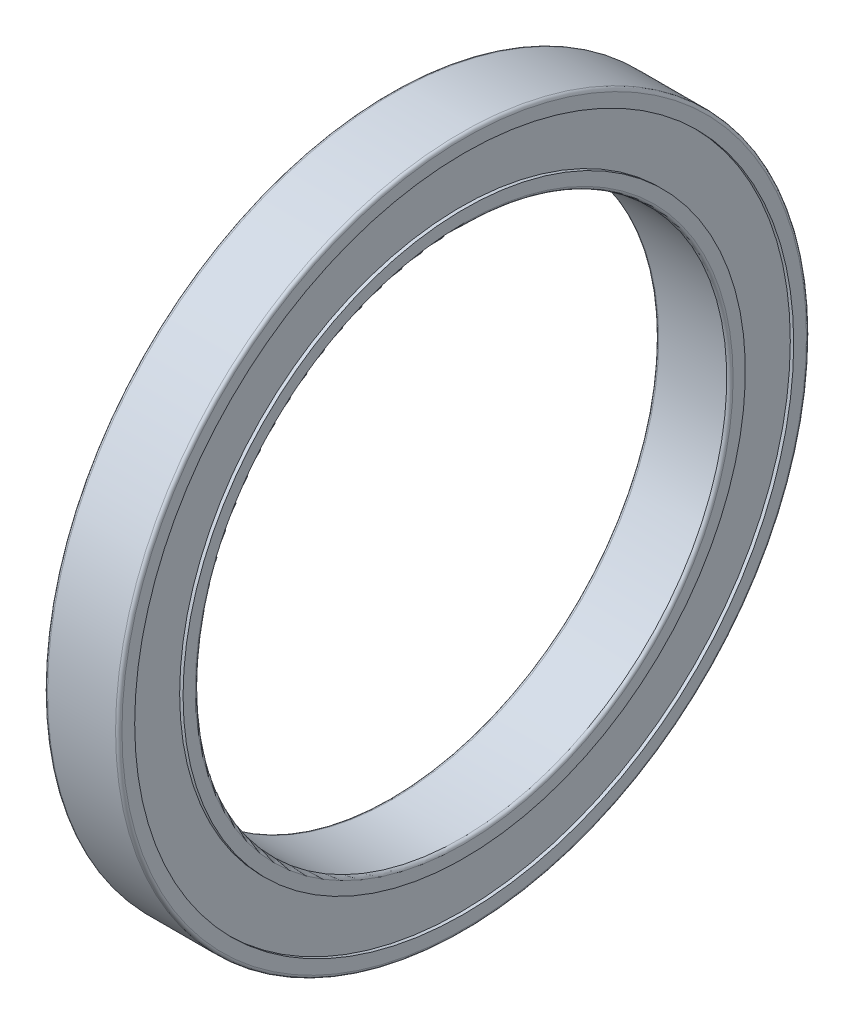
SolidWorks part; units mm, degrees
ref_plane "Front Plane" through (0, 0, 0) normal (0, 0, 1) x (1, 0, 0)
ref_plane "Top Plane" through (0, 0, 0) normal (0, 1, 0) x (1, 0, 0)
ref_plane "Right Plane" through (0, 0, 0) normal (1, 0, 0) x (0, 0, -1)
sketch "Sketch1" plane through (0, 0, 0) normal (0, 0, 1) x (1, 0, 0)
  line L0 (0, 0) -> (7, 0) construction
  line L1 (0, 25) -> (7, 25)
  line L2 (0, 32.5) -> (7, 32.5)
  line L3 (0, 32.5) -> (0, 31)
  line L4 (0, 31) -> (0.32, 31)
  line L5 (7, 32.5) -> (7, 31)
  line L6 (0.32, 31) -> (0.32, 26.45)
  line L7 (0.32, 26.45) -> (0, 26.45)
  line L8 (0, 26.45) -> (0, 25)
  line L9 (7, 31) -> (6.68, 31)
  line L10 (6.68, 31) -> (6.68, 26.45)
  line L11 (6.68, 26.45) -> (7, 26.45)
  line L12 (7, 26.45) -> (7, 25)
  dimension "D" = 65
  dimension "B" = 7
  dimension "D_s" = 50
  dimension "MSM_1" = 62
  dimension "MSM_2" = 52.9
  dimension "MSM_3" = 0.32
revolve "Revolve1" add sketch "Sketch1" angle 360 about L0
fillet "Fillet1" radius 0.3 2 edges at (7, 0, 32.5) (0, 0, 32.5)
fillet "Fillet2" radius 0.3 2 edges at (7, 0, 25) (0, 0, 25)
